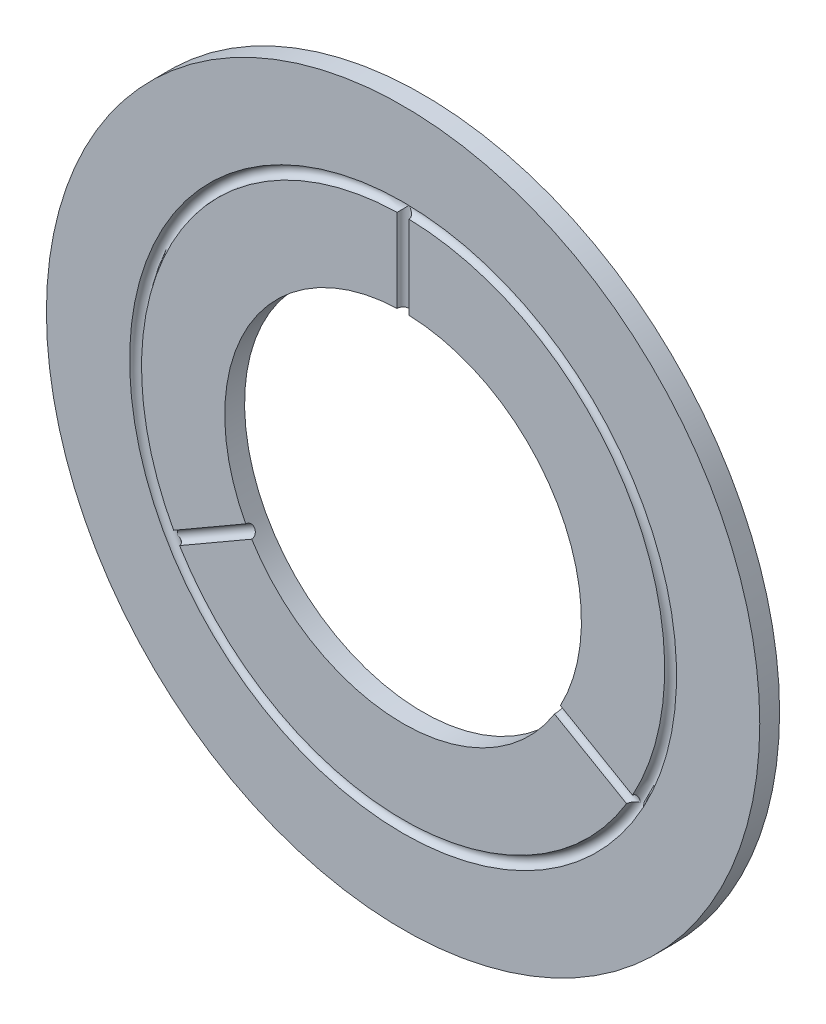
from build123d import *

# Parameters (mm, degrees)
SKETCH_1_R               = 90
SKETCH_1_R_2             = 45
EXTRUDE_1_DEPTH          = 5
SKETCH_3_R               = 1.5
SKETCH_5_R               = 1.5
CUT_EXTRUDE_2_DEPTH      = 67.5
PATTERN_CIRCULAR_1_COUNT = 3


with BuildPart() as part:
    # 草图1 → 凸台-拉伸1 (new body)
    with BuildSketch(Plane.XY):
        Circle(SKETCH_1_R)
        Circle(SKETCH_1_R_2, mode=Mode.SUBTRACT)
    extrude(amount=EXTRUDE_1_DEPTH)

    # 切除-扫描1: sweep along a path in 草图2
    with BuildLine(Plane.XY.offset(5)) as sweep_1_path:
        CenterArc((0, 0), 67.5, 0, 360)
    # 草图3 → 切除-扫描1 (sweep, cut)
    with BuildSketch(Plane(origin=(0, 0, 0), x_dir=(0, 0, -1), z_dir=(1, 0, 0))):
        with Locations((-5, 67.5)):
            Circle(SKETCH_3_R)
    sweep(path=sweep_1_path.line, mode=Mode.SUBTRACT)

    # 草图5 → 切除-拉伸2 (cut)
    with BuildSketch(Plane(origin=(0, 0, 0), x_dir=(1, 0, 0), z_dir=(0, 1, 0))):
        with Locations((0, -5)):
            Circle(SKETCH_5_R)
    cut_extrude_2 = extrude(amount=CUT_EXTRUDE_2_DEPTH, mode=Mode.SUBTRACT)

    # 阵列(圆周)1: 切除-拉伸2 ×3 about axis
    pattern_circular_1_axis = Axis((0, 0, 5), (0, 0, -1))
    for i in range(1, PATTERN_CIRCULAR_1_COUNT):
        add(cut_extrude_2.rotate(pattern_circular_1_axis, i * 360 / PATTERN_CIRCULAR_1_COUNT), mode=Mode.SUBTRACT)


solid = part.part
